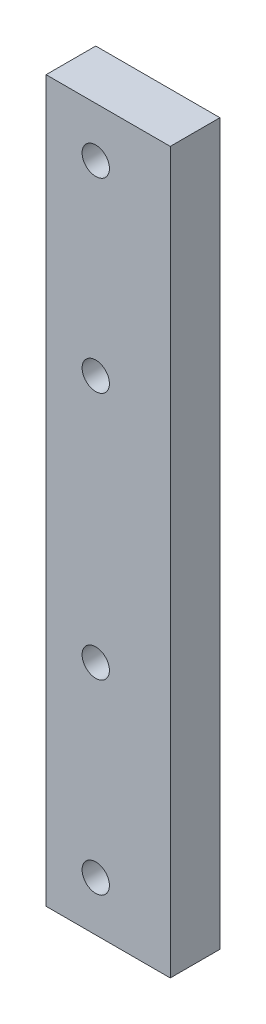
SolidWorks part; units mm, degrees
ref_plane "前视基准面" through (0, 0, 0) normal (0, 0, 1) x (1, 0, 0)
ref_plane "上视基准面" through (0, 0, 0) normal (0, 1, 0) x (1, 0, 0)
ref_plane "右视基准面" through (0, 0, 0) normal (1, 0, 0) x (0, 0, -1)
other "Configuration Table"
sketch "草图1" plane through (0, 0, 0) normal (0, 0, 1) x (1, 0, 0)
  line L1 (-25, -145) -> (25, -145)
  line L2 (-25, -145) -> (-25, 145)
  line L3 (-25, 145) -> (25, 145)
  line L4 (25, -145) -> (25, 145)
  line L5 (0, 145) -> (0, -145) construction
  line L6 (-25, 0) -> (25, 0) construction
  point P0 (0, 0)
  dimension "D1" = 290
  dimension "D2" = 50
extrude "凸台-拉伸1" add sketch "草图1" along normal blind 20
sketch "草图4" plane through (0, 0, 20) normal (0, 0, 1) x (1, 0, 0)
  line L0 (25, 145) -> (-25, 145) construction
  line L1 (-25, 145) -> (-25, -145) construction
  point P0 (-5, 125)
  point P2 (-5, 50)
  point P4 (-5, -50)
  point P6 (-5, -125)
  dimension "D1" = 20
  dimension "D2" = 20
  dimension "D3" = 75
  dimension "D4" = 20
  dimension "D5" = 100
  dimension "D6" = 20
  dimension "D7" = 20
  dimension "D8" = 75
hole_wizard "Ø11.0 (11) 直径孔1" positions "草图4" profile "草图3" hole size "Ø11.0" standard "GB"
sketch "草图3" plane through (-5, 125, 20) normal (1, 0, 0) x (0, -1, 0)
  line L0 (0, 0) -> (0, 39.3047)
  line L1 (0, 39.3047) -> (5.5, 36)
  line L2 (5.5, 36) -> (5.5, 0)
  line L5 (5.5, 0) -> (0, 0)
  line L10 (0, 39.3047) -> (-5.5, 36) construction
  line L11 (0, -6.35) -> (0, 107.95) construction
  dimension "孔直径" = 11
  dimension "孔深度" = 36
  dimension "导头角度" = 118
